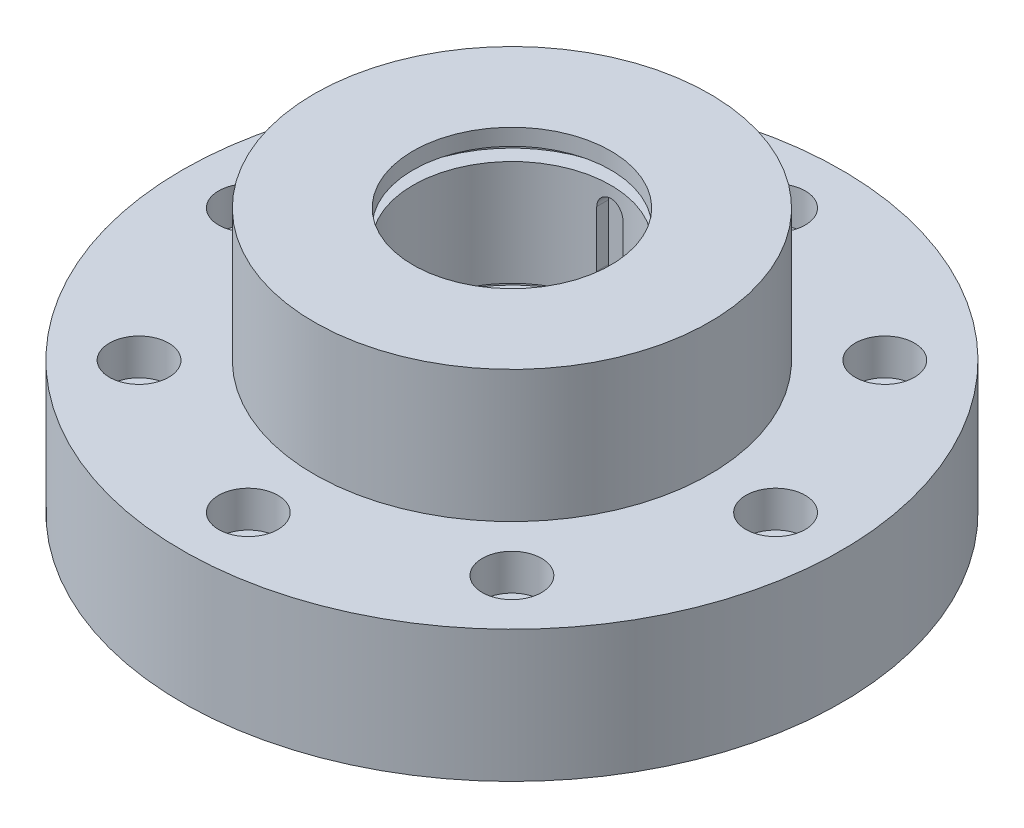
SolidWorks part; units mm, degrees
ref_plane "前视基准面" through (0, 0, 0) normal (0, 0, 1) x (1, 0, 0)
ref_plane "上视基准面" through (0, 0, 0) normal (0, 1, 0) x (1, 0, 0)
ref_plane "右视基准面" through (0, 0, 0) normal (1, 0, 0) x (0, 0, -1)
sketch "草图1" plane through (0, 0, 0) normal (0, 0, 1) x (1, 0, 0)
  line L0 (0, 82.6364) -> (0, -118.6364) construction
  line L1 (30, 64.0909) -> (60, 64.0909)
  line L2 (60, 64.0909) -> (60, 24.0909)
  line L3 (60, 24.0909) -> (100, 24.0909)
  line L4 (100, 24.0909) -> (100, -15.9091)
  line L5 (100, -15.9091) -> (57.5, -15.9091)
  line L6 (57.5, -15.9091) -> (57.5, -35.9091)
  line L7 (57.5, -35.9091) -> (40, -35.9091)
  line L8 (40, -35.9091) -> (40, -5.9091)
  line L9 (40, -5.9091) -> (35, -5.9091)
  line L10 (35, -5.9091) -> (35, 14.0909)
  line L11 (35, 14.0909) -> (30, 14.0909)
  line L12 (30, 14.0909) -> (30, 19.0909)
  line L13 (30, 19.0909) -> (35, 19.0909)
  line L14 (35, 19.0909) -> (35, 23.0909)
  line L15 (35, 23.0909) -> (30, 23.0909)
  line L16 (30, 23.0909) -> (30, 55.0909)
  line L17 (30, 55.0909) -> (35, 55.0909)
  line L18 (35, 55.0909) -> (35, 59.0909)
  line L19 (35, 59.0909) -> (30, 59.0909)
  line L20 (30, 59.0909) -> (30, 64.0909)
  dimension "D1" = 30
  dimension "D2" = 30
  dimension "D3" = 30
  dimension "D4" = 40
  dimension "D5" = 42.5
  dimension "D6" = 17.5
  dimension "D7" = 5
  dimension "D8" = 30
  dimension "D9" = 5
  dimension "D10" = 5
  dimension "D11" = 5
  dimension "D12" = 30
  dimension "D13" = 20
  dimension "D14" = 4
  dimension "D15" = 32
  dimension "D16" = 4
  dimension "D17" = 40
  dimension "D18" = 40
  dimension "D19" = 20
revolve "旋转1" add sketch "草图1" angle 360 about L0
sketch "草图2" plane through (0, 24.0909, 0) normal (0, 1, 0) x (1, 0, 0)
  circle A0 centre (80, 0) radius 9
  circle A1 centre (56.5685, -56.5685) radius 9
  circle A2 centre (0, -80) radius 9
  circle A3 centre (-56.5685, -56.5685) radius 9
  circle A4 centre (-80, 0) radius 9
  circle A5 centre (-56.5685, 56.5685) radius 9
  circle A6 centre (0, 80) radius 9
  circle A7 centre (56.5685, 56.5685) radius 9
  point P19 (0, 0)
  dimension "D1" = 18
  dimension "D2" = 80
  dimension "D3" = 8
extrude "切除-拉伸1" cut sketch "草图2" against normal blind 11
sketch "草图3" plane through (0, 13.0909, 0) normal (0, 1, 0) x (1, 0, 0)
  circle A0 centre (56.5685, 56.5685) radius 5.25
  circle A1 centre (80, 0) radius 5.25
  circle A2 centre (56.5685, -56.5685) radius 5.25
  circle A3 centre (0, -80) radius 5.25
  circle A4 centre (-56.5685, -56.5685) radius 5.25
  circle A5 centre (-80, 0) radius 5.25
  circle A6 centre (-56.5685, 56.5685) radius 5.25
  circle A7 centre (0, 80) radius 5.25
  point P19 (0, 0)
  dimension "D1" = 10.5
  dimension "D2" = 8
extrude "切除-拉伸2" cut sketch "草图3" against normal up to next
sketch "草图4" plane through (0, 0, 0) normal (1, 0, 0) x (0, 0, -1)
  line L0 (0, 96.6887) -> (0, -123.3699) construction
ref_plane "基准面1" through (0, 0, 0) normal (0.9239, 0, 0.3827) x (0, -1, 0)
sketch "草图5" plane through (0, 0, 0) normal (0.9239, 0, 0.3827) x (0, -1, 0)
  line L0 (-4.0909, 122.9192) -> (-4.0909, 3.6221) construction
  line L1 (-4.0909, 100) -> (5.9091, 100)
  line L2 (15.9091, 100) -> (-24.0909, 100) construction
  line L3 (5.9091, 100) -> (0.8502, 84.4303)
  line L5 (-4.0909, 0) -> (-4.0909, -30.2527) construction
  line L6 (-96.6887, 0) -> (123.3699, 0) construction
  line L7 (-4.0909, 3.6221) -> (-4.0909, 100)
  line L8 (-4.0909, 3.6221) -> (0.8502, 3.6221)
  line L9 (0.8502, 3.6221) -> (0.8502, 84.4303)
  dimension "D1" = 10
  dimension "D2" = 4.9411
  dimension "D3" = 18
revolve "切除-旋转1" cut sketch "草图5" angle 360 about L0
sketch "草图6" plane through (0, 55.0909, 0) normal (0, 1, 0) x (1, 0, 0)
  line L0 (0, 147.1352) -> (0, -143.2557) construction
  line L1 (-4, 29.7321) -> (4, 29.7321) construction
  line L2 (-4, 33.2321) -> (4, 33.2321)
  line L3 (-4, 33.2321) -> (-4, 26.2321)
  line L4 (-4, 26.2321) -> (4, 26.2321)
  line L5 (4, 33.2321) -> (4, 26.2321)
  line L6 (-4, 33.2321) -> (4, 26.2321) construction
  line L7 (-4, 26.2321) -> (4, 33.2321) construction
  circle A1 centre (0, 0) radius 30 construction
  point P3 (0, 29.7321)
  dimension "D3" = 60
  dimension "D1" = 7
  dimension "D2" = 8
  dimension "D4" = 8
  dimension "D5" = 3.5
extrude "切除-拉伸3" cut sketch "草图6" against normal blind 17 from offset 7.5 offset against normal yes
sketch "草图7" plane through (0, 0, -33.2321) normal (0, 0, 1) x (1, 0, 0)
  line L5 (-4, 30.5909) -> (4, 30.5909)
  line L6 (-4, 47.5909) -> (-4, 30.5909)
  line L7 (4, 47.5909) -> (-4, 47.5909)
  line L8 (4, 30.5909) -> (4, 47.5909)
  line L9 (-4, 30.5909) -> (4, 30.5909)
  line L10 (-4, 47.5909) -> (-4, 30.5909)
  line L11 (4, 47.5909) -> (-4, 47.5909)
  line L12 (4, 30.5909) -> (4, 47.5909)
  arc A0 (-4, 47.5909) -> (4, 47.5909) centre (0, 47.5909) cw
  arc A1 (-4, 30.5909) -> (4, 30.5909) centre (0, 30.5909) ccw
  line M5 (4, 47.5909) -> (-4, 47.5909)
  line M7 (-4, 30.5909) -> (4, 30.5909)
  dimension "D1" = 0
extrude "切除-拉伸4" cut sketch "草图7" along normal blind 7 contours A0 M5 | A1 M7
